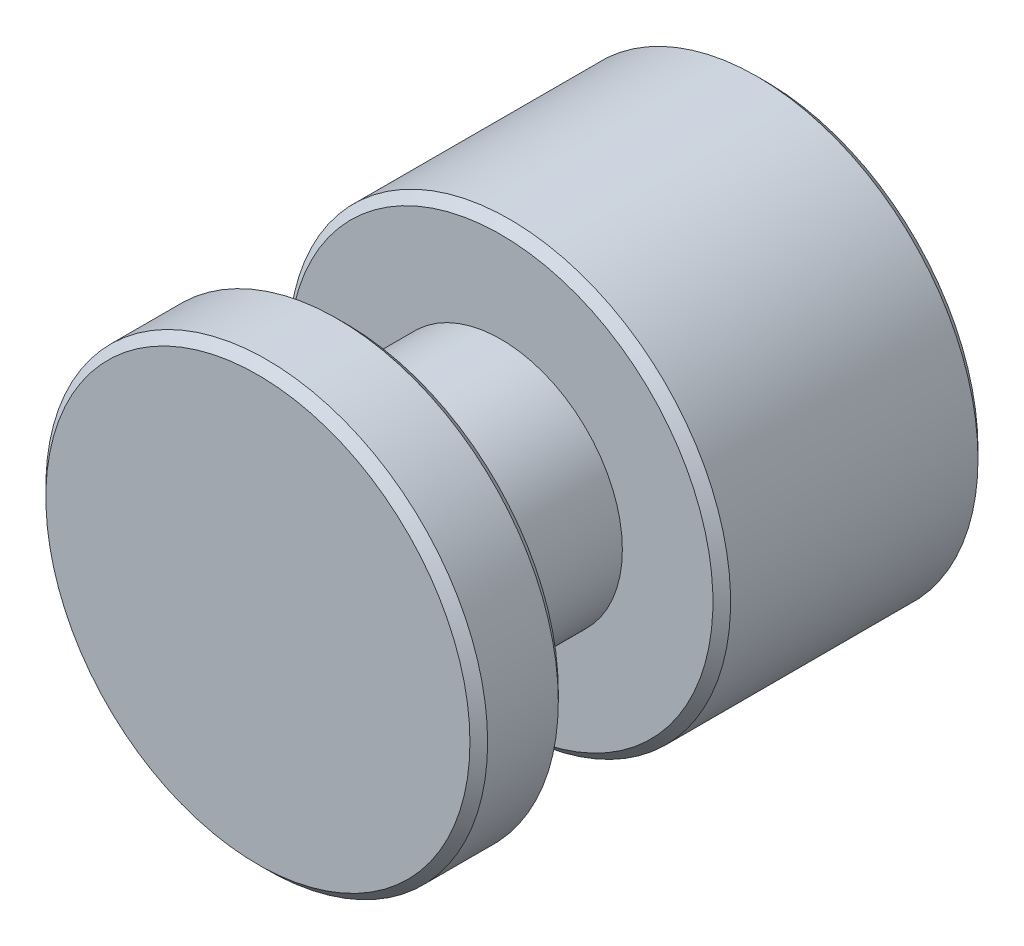
SolidWorks part; units mm, degrees
material "Alloy steel"
ref_plane "Front Plane" through (0, 0, 0) normal (0, 0, 1) x (1, 0, 0)
ref_plane "Top Plane" through (0, 0, 0) normal (0, 1, 0) x (1, 0, 0)
ref_plane "Right Plane" through (0, 0, 0) normal (1, 0, 0) x (0, 0, -1)
sketch "Sketch1" plane through (0, 0, 0) normal (0, 0, 1) x (1, 0, 0)
  circle A0 centre (0, 0) radius 5
  dimension "D1" = 10
extrude "Boss-Extrude1" add sketch "Sketch1" along normal blind 6
sketch "Sketch2" plane through (0, 0, 6) normal (0, 0, 1) x (1, 0, 0)
  circle A0 centre (0, 0) radius 2.75
  dimension "D1" = 5.5
extrude "Boss-Extrude2" add sketch "Sketch2" along normal blind 3.5
sketch "Sketch3" plane through (0, 0, 9.5) normal (0, 0, 1) x (1, 0, 0)
  circle A0 centre (0, 0) radius 5
  dimension "D1" = 10
extrude "Boss-Extrude3" add sketch "Sketch3" along normal blind 2
hole_wizard "M4 tapped hole1" positions "Sketch5" profile "Sketch4" tap size "M4" standard "Iso"
sketch "Sketch5" plane through (0, 0, 0) normal (0, 0, -1) x (-1, 0, 0)
  point P0 (0, 0)
sketch "Sketch4" plane through (0, 0, 0) normal (1, 0, 0) x (0, 1, 0)
  line L0 (0, 0) -> (0, 8.9914)
  line L1 (0, 8.9914) -> (1.65, 8)
  line L2 (1.65, 8) -> (1.65, 0)
  line L5 (1.65, 0) -> (0, 0)
  line L10 (0, 8.9914) -> (-1.65, 8) construction
  line L11 (0, -6.35) -> (0, 107.95) construction
  dimension "螺孔鑽直徑" = 3.3
  dimension "螺孔鑽深度" = 8
  dimension "導頭角度" = 118
cosmetic thread "Cosmetic thread1" parameters "D1"=6, "D2"=4
chamfer "Chamfer1" distance 0.2 angle 45 4 edges at (5, 0, 0) (5, 0, 6) (5, 0, 9.5) (5, 0, 11.5)
